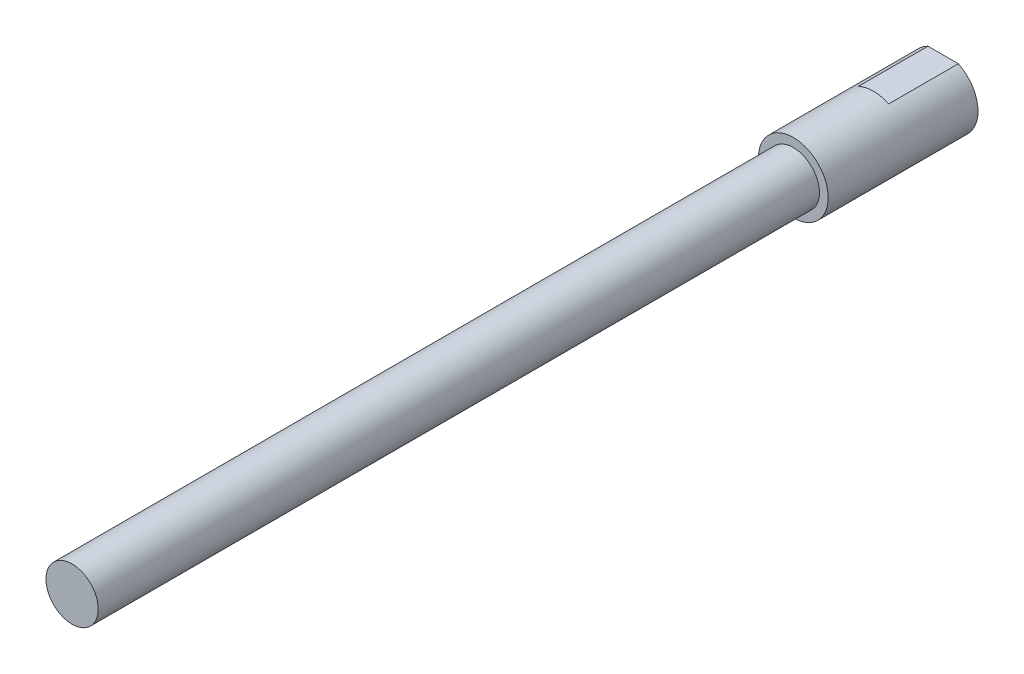
SolidWorks part; units mm, degrees
ref_plane "前视基准面" through (0, 0, 0) normal (0, 0, 1) x (1, 0, 0)
ref_plane "上视基准面" through (0, 0, 0) normal (0, 1, 0) x (1, 0, 0)
ref_plane "右视基准面" through (0, 0, 0) normal (1, 0, 0) x (0, 0, -1)
sketch "草图1" plane through (0, 0, 0) normal (0, 0, 1) x (1, 0, 0)
  circle A0 centre (0, 0) radius 7.5
  dimension "D1" = 15
extrude "凸台-拉伸1" add sketch "草图1" along normal blind 207
sketch "草图2" plane through (0, 0, 0) normal (0, 0, -1) x (-1, 0, 0)
  circle A0 centre (0, 0) radius 10
  dimension "D1" = 20
extrude "凸台-拉伸2" add sketch "草图2" along normal blind 43
sketch "草图3" plane through (0, 0, -43) normal (0, 0, -1) x (-1, 0, 0)
  line L1 (-11.5, -9) -> (11.5, -9)
  line L2 (-11.5, -9) -> (-11.5, 9)
  line L3 (-11.5, 9) -> (11.5, 9)
  line L4 (11.5, -9) -> (11.5, 9)
  line L5 (-11.5, -9) -> (11.5, 9) construction
  line L6 (-11.5, 9) -> (11.5, -9) construction
  point P0 (0, 0)
  dimension "D1" = 18
  dimension "D2" = 23
extrude "切除-拉伸1" cut sketch "草图3" against normal blind 20 flip side to cut
hole_wizard "M8 螺纹孔1" positions "3D草图1" profile "草图4" tap size "M8" standard "GB"
sketch3d "3D草图1"
  arc A0 (-4.3589, -9, -43) -> (-4.3589, 9, -43) centre (0, 0, -43) ccw construction
  point P0 (0, 0, -43)
  point P6 (0, 0, -53)
sketch "草图4" plane through (0, 0, -43) normal (1, 0, 0) x (0, 1, 0)
  line L0 (0, 0) -> (0, 20.2929)
  line L1 (0, 20.2929) -> (3.4, 18.25)
  line L2 (3.4, 18.25) -> (3.4, 0.625)
  line L3 (3.4, 0.625) -> (4.025, 0)
  line L5 (4.025, 0) -> (0, 0)
  line L6 (-3.4, 0.625) -> (-4.025, 0) construction
  line L10 (0, 20.2929) -> (-3.4, 18.25) construction
  line L11 (0, -6.35) -> (0, 107.95) construction
  dimension "螺纹孔钻头直径" = 6.8
  dimension "螺纹孔钻头深度" = 18.25
  dimension "近端锥形沉头孔直径" = 8.05
  dimension "近端锥形沉头孔角度" = 90
  dimension "导头角度" = 118
cosmetic thread "孔螺蚊线1"
